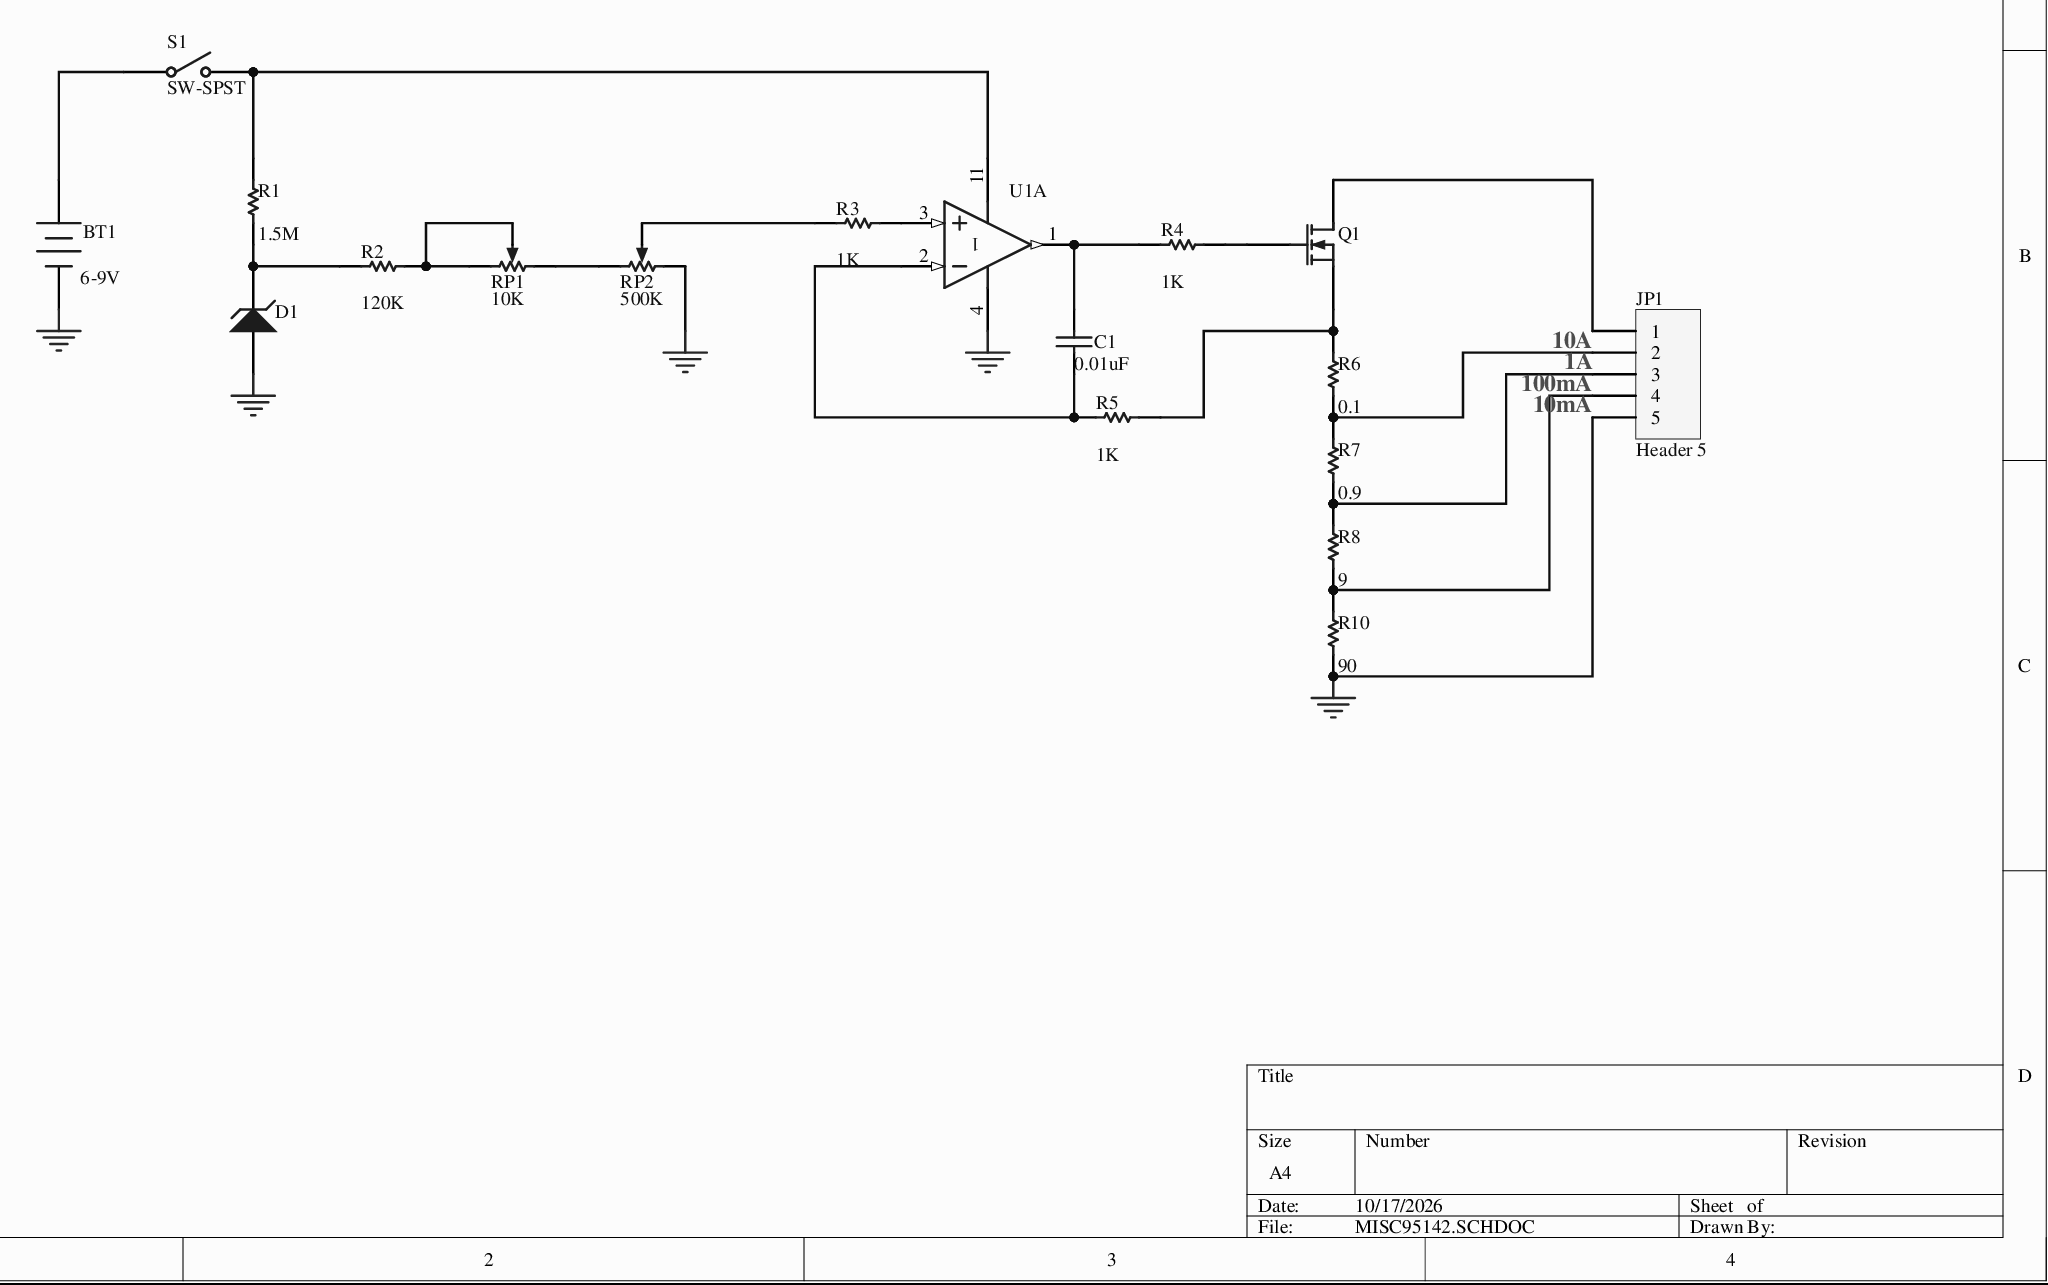
[diagram p0: MISC95142.SCHDOC]
# Altium project MISC95142.PRJPCB
1 sheet, 18 parts. Net scope: global (net labels, ports and power ports of the same name join across sheets).
Board file: MISC95142.PCBDOC

## Sheet MISC95142.SCHDOC
size A4

### Parts
BT1  Battery  [BAT-2]  (value not drawn)
C1  value 0.01uF  [RAD-0.3]  (hidden comment: Cap)
D1  D Zener  [DIODE-0.7]  (value not drawn)
JP1  Header 5  [HDR1X5]
Q1  MOSFET-N  [BCY-W3/H.8]  (value not drawn)
R1  value 1.5M  [AXIAL-0.3]  (hidden comment: Res1)
R2  value 120K  [AXIAL-0.3]  (hidden comment: Res1)
R3  value 1K  [AXIAL-0.3]  (hidden comment: Res1)
R4  value 1K  [AXIAL-0.3]  (hidden comment: Res1)
R5  value 1K  [AXIAL-0.3]  (hidden comment: Res1)
R6  value 0.1  [AXIAL-0.3]  (hidden comment: Res1)
R7  value 0.9  [AXIAL-0.3]  (hidden comment: Res1)
R8  value 9  [AXIAL-0.3]  (hidden comment: Res1)
R10  value 90  [AXIAL-0.3]  (hidden comment: Res1)
RP1  value 10K  [VR2]  (hidden comment: RPot)
RP2  value 500K  [VR2]  (hidden comment: RPot)
S1  SW-SPST  [SPST-2]
U1  LM248J  [J014]  (value not drawn)  (part A of 4)

### Nets
GND: BT1.2(-) D1.1(A) JP1.5 R10.1 RP2.1(TOP) U1.4(V+)
NetBT1_1: BT1.1(+) S1.1(COMMON)
NetC1_1: C1.1 R5.1 U1.2(IN-)
NetC1_2: C1.2 R4.1 U1.1(OUT)
NetD1_2: D1.2(K) R1.1 R2.1
NetJP1_1: JP1.1 Q1.1(D)
NetJP1_2: JP1.2 R6.1 R7.2
NetJP1_3: JP1.3 R7.1 R8.2
NetJP1_4: JP1.4 R8.1 R10.2
NetQ1_2: Q1.2(G) R4.2
NetQ1_3: Q1.3(S) R5.2 R6.2
NetR1_2: R1.2 S1.2(NO) U1.11(V-)
NetR2_2: R2.2 RP1.2(BOT) RP1.3(TAP)
NetR3_1: R3.1 RP2.3(TAP)
NetR3_2: R3.2 U1.3(IN+)
NetRP1_1: RP1.1(TOP) RP2.2(BOT)

### Notes on the sheet
- (near JP1) 10A
- (near JP1) 1A
- (near JP1) 100mA
- (near JP1) 10mA

### Library data of the parts
BT1 = Battery: Multicell Battery; Published: 24-Mar-1999; Revision: July-2002: Re-released for DXP Platform.; Publisher: Altium Limited
C1 = Cap: Capacitor; Published: 8-Jun-2000; Revision: July-2002: Re-released for DXP Platform.; Publisher: Altium Limited
D1 = D Zener: Zener Diode; Published: 8-Jun-2000; Revision: July-2002: Re-released for DXP Platform.; Publisher: Altium Limited
JP1 = Header 5: Header, 5-Pin; Revision: 17-Jul-2002: Re-released for DXP Platform.; Publisher: Altium Limited
Q1 = MOSFET-N: N-Channel MOSFET; Published: 8-Jun-2000; Revision: July-2002: Re-released for DXP Platform.; Publisher: Altium Limited
R1-R8 R10 = Res1: Resistor; Published: 8-Jun-2000; Revision: July-2002: Re-released for DXP Platform.; Publisher: Altium Limited
RP1 RP2 = RPot: Potentiometer; Set Position: 0.5; Published: 8-Jun-2000; Revision: July-2002: Re-released for DXP Platform.; Publisher: Altium Limited
S1 = SW-SPST: Single-Pole, Single-Throw Switch; Published: 24-Mar-1999; Revision: July-2002: Re-released for DXP Platform.; Publisher: Altium Limited
U1 = LM248J: Quadruple Operational Amplifier; Package Information: Latest Revision: Jun-1999; Published: 15-Apr-2002; Datasheet: Linear Circuits Data Book 1989 Volume 1 (Mar-1988); Package Reference: J014; Publisher: Altium Limited